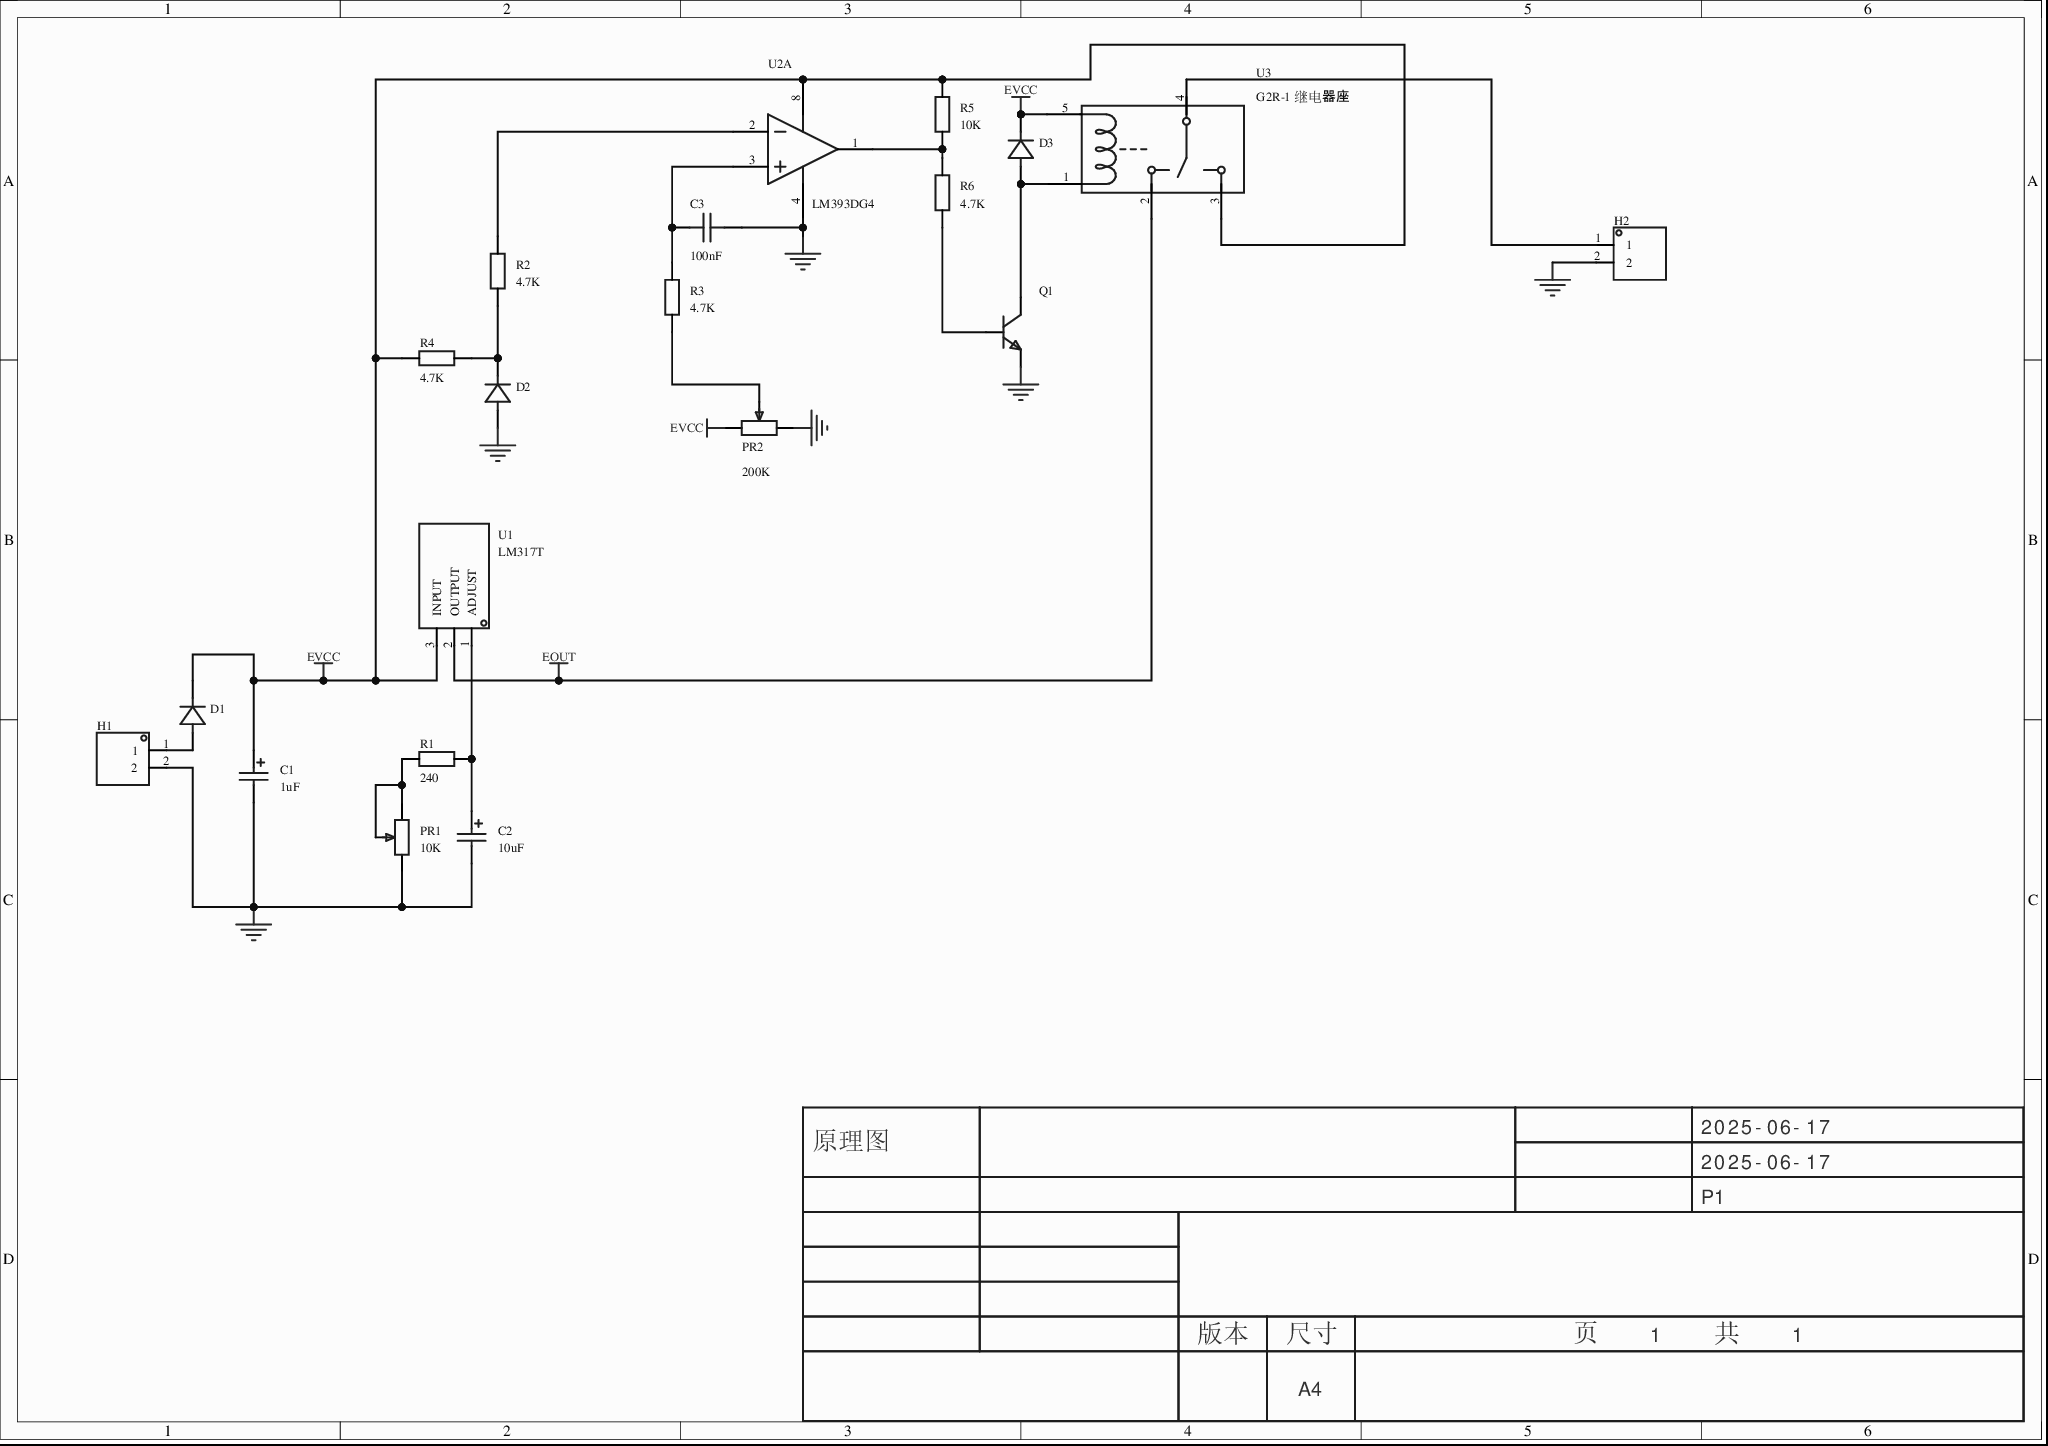
[diagram p0: MISC52117-3.schdoc]
# Altium project MISC52117-2.PrjPcb
1 sheet, 20 parts. Net scope: global (net labels, ports and power ports of the same name join across sheets).
Board file: MISC52117.pcbdoc

## Sheet MISC52117-3.schdoc
size 297 x 209 mm; Version: V1.0; @Project Name: MISC52117; @Page Count: 1; @Update Date: 2025-06-17; @Create Date: 2025-06-17; @Schematic Name: MISC52117; @Page No: 1; @Create Time: 08:55:39; @Update Time: 08:55:39; @Board Name: MISC52117

### Parts
C1  1uF  [C_Ele_SMD_3x5.4mm]
C2  10uF  [C_Ele_SMD_3x5.4mm]
C3  100nF  [C0603]
D1  (no value)  [DO_1N4007]
D2  (no value)  [DO_1N4007]
D3  (no value)  [DO_1N4007]
H1  (no value)  [HDR-TH_2P-P2.54-V-M-1]
H2  (no value)  [HDR-TH_2P-P2.54-V-M-1]
PR1  10K  [R_3386P]
PR2  200K  [R_3386P]
Q1  (no value)  [S8050_SOT-23]
R1  240  [R0603]
R2  4.7K  [R0603]
R3  4.7K  [R0603]
R4  4.7K  [R0603]
R5  10K  [R0603]
R6  4.7K  [R0603]
U1  LM317T  [TO-220-3_L10.2-W4.6-P2.54-L]
U2  LM393DG4  [SOIC-8_L4.9-W3.9-P1.27-LS6.0-BL]  (part A of 2)
U3  G2R-1 继电器座  [RELAY-TH_G2R-1_C9900014679]

### Nets
EOUT: U1.2(OUTPUT) U3.2
EVCC: C1.1 D1.1(K) D3.1(K) PR2.3 R4.2 R5.2 U1.3(INPUT) U2.8(VDD) U3.3 U3.5
GND: C1.2 C2.2 C3.2 D2.2(A) H1.2 H2.2 PR1.3 PR2.1 Q1.2 U2.4(GND)
NetC2_1: C2.1 R1.2 U1.1(ADJUST)
NetC3_1: C3.1 R3.2 U2.3(1IN+)
NetD1_2: D1.2(A) H1.1
NetD2_1: D2.1(K) R2.1 R4.1
NetD3_2: D3.2(A) Q1.3 U3.1
NetH2_1: H2.1 U3.4
NetPR1_1: PR1.1 PR1.2 R1.1
NetPR2_2: PR2.2 R3.1
NetQ1_1: Q1.1 R6.1
NetR2_2: R2.2 U2.2(1IN-)
NetR5_1: R5.1 R6.2 U2.1(1OUT)

### Notes on the sheet
- 2025-06-17
- 原理图
- P1
- 版本
- 尺寸
- A4
- 页    1    共    1

### Library data of the parts
C1 C2 = C_Ele_SMD_3x5.4mm: Symbol: CAP; AddInBom: yes; ModelId: 0132c3d3fdbf4fd987f710a97e7a5b5d; ModelName: CAP-SMD_BD3.0-L3.3-W3.3-H5.3; ModelTransform: 129.9,149.58,209.06,-90,0,0,0,0,0; Device: C_Ele_SMD_3x5.4mm; Supplier Footprint: SMD,3x5.4mm; ConvertToPcb: yes; FootprintName: C_Ele_SMD_3x5.4mm
  C1: Value: 1uF
  C2: Value: 10uF
C3 = CAP_0603: ConvertToPcb: yes; SymbolName: CapAcitance; ModelId: ac125912035d415993ca9572d50418b1; ModelName: C0603_L1.6-W0.8-H0.8; ModelTransform: 62.992,31.496,0,0,0,0,0,0,0; Device: CAP_0603; AddInBom: yes; Supplier Footprint: 0603; FootprintName: C0603; Value: 100nF
D1-D3 = D_1N4007A: AddInBom: yes; ModelId: 6de1e9b71a0d4751b4e9df530304c1a3; ModelName: DO-41_D2.4-L4.7-P8.70; ModelTransform: 373.9,94.4,232.29,0,0,0,0,0,-140; Symbol: D_1N4007; Device: D_1N4007A; Supplier Footprint: DO-41; ConvertToPcb: yes; FootprintName: DO_1N4007
H1 H2 = HDR-M_2.54_1x2P: Symbol: 210S-1*2P L=11.6MMGold-plated black; ConvertToPcb: yes; ModelId: 79b2e9f2d70a4d68a1b7098f27c6d4c5; ModelName: HDR-M-2.54_1x2; ModelTransform: 200,100,0,0,0,0,0,0,-118.11; Device: HDR-M_2.54_1x2P; AddInBom: yes; SupplierPart: C124375; Supplier Footprint: 插件; FootprintName: HDR-TH_2P-P2.54-V-M-1
PR1 PR2 = R_3386P: Symbol: 3386P-1-103LF; ConvertToPcb: yes; ModelId: 6a25d8a4450b4318959c1cd98efa6b0c0819f05c4eef4c71ace90d822a990e87; ModelName: RES-ADJ-TH_3P-L9.5-W9.5-P2.54-BR-BS; ModelTransform: 375.19,375.19,387,-90,0,0,0,0,-197; Device: R_3386P; AddInBom: yes; FootprintName: R_3386P; Supplier Footprint: 直插
  PR1: Value: 10K
  PR2: Value: 200K
Q1 = S8050_SOT_NPN: ConvertToPcb: yes; SymbolName: NPN; ModelId: c62791f0466c4ae2a892c056b845b0ca; ModelName: SOT-23-3P_L2.9-W1.3-H1.0-LS2.4-P0.95; ModelTransform: 98.6,114.12,41.29,180,0,0,0,0,-3; Device: S8050_SOT_NPN; AddInBom: yes; Supplier Footprint: SOT-23; FootprintName: S8050_SOT-23
R1-R6 = Res_0603: ConvertToPcb: yes; SymbolName: 电阻; ModelId: fc143cca1e79419f9cd78b61e9279f08; ModelTransform: 31.8897,63.7794,0,90,0,0,0,0,0; Device: Res_0603; AddInBom: yes; Supplier Footprint: 0603; FootprintName: R0603; ModelName: R0603
  R1: Value: 240
  R2-R4 R6: Value: 4.7K
  R5: Value: 10K
U1 = LM317T: 输出类型:可调;最大输入电压:40V;输出电压:1.2V~37V;输出电流:1.5A;电源纹波抑制比(PSRR):-;输出极性:正极;; Manufacturer: UMW(友台半导体); Symbol: LM317T_C3014307; AddInBom: yes; ModelId: 6197bb0aad96481ab8a17aa6d23d90f1; ModelTransform: 399.999,177.204,0,0,0,0,0,24.606,-196.85; Output Type: 可调; Maximum Input Voltage: 40V; Output Current: 1.5A; standby current: 12mA; Output Polarity: 正极; Number of Outputs: 1; Device: LM317T; LCSC Part Name: LM317T; SupplierPart: C3014307; ManufacturerPart: LM317T; Supplier Footprint: TO-220; JLCPCB Part Class: 扩展库; Datasheet: https://atta.szlcsc.com/upload/public/pdf/source/20241113/1F0111AE0226A3AB59038DF856FC50AF.pdf; Supplier: LCSC; ConvertToPcb: yes; FootprintName: TO-220-3_L10.2-W4.6-P2.54-L; ModelName: TO-220-3_L10.2-W4.6-P2.54-L; Output Voltage: 1.2V~37V; Power Supply Rejection Ratio (PSRR): -; Dropout Voltage: -; Noise: -; Feature: 过流保护(OCP)；短路保护；热保护(TSD); Operating Temperature: -40℃~+125℃@(Tj)
U2 = LM393DG4: Manufacturer: TI(德州仪器); Relevance: []; AddInBom: yes; ModelId: e81d2f7d937b4a6ab1dca543ff5d56a4; ModelName: SOIC-8_L4.9-W3.9-H1.7-LS6.0-P1.27; ModelTransform: 189.751,236.22,0,0,0,0,0.0005,0.0005,0; Symbol: LM393DG4; Device: LM393DG4; LCSC Part Name: LM393DG4; SupplierPart: C3658999; ManufacturerPart: LM393DG4; Supplier Footprint: SOIC-8; JLCPCB Part Class: 扩展库; Datasheet: https://www.ti.com/cn/lit/gpn/lm393a; Supplier: LCSC; ConvertToPcb: yes; FootprintName: SOIC-8_L4.9-W3.9-P1.27-LS6.0-BL
U3 = G2R-1 继电器座: AddInBom: yes; ModelId: e79d4cd8b15746fc8477b7b7b5cbc961; ModelTransform: 1141.73,499.999,0,0,0,0,25,-0.591,-157.48; Symbol: G2R-1 继电器座; Device: G2R-1 继电器座; LCSC Part Name: G2R-1 继电器座; SupplierPart: C9900014679; ManufacturerPart: G2R-1 继电器座; Supplier Footprint: G2R-1; JLCPCB Part Class: 扩展库; Supplier: LCSC; ConvertToPcb: yes; FootprintName: RELAY-TH_G2R-1_C9900014679; ModelName: RELAY-TH_G2R-1_C9900014679